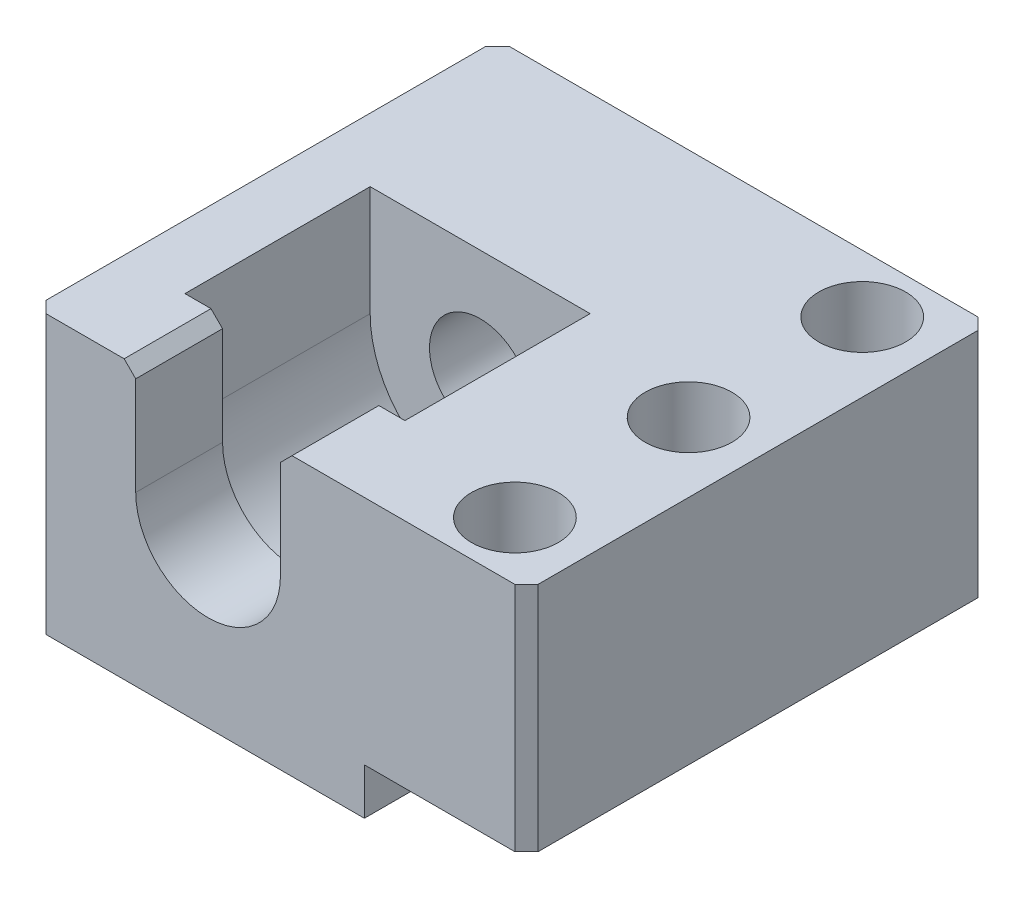
SolidWorks part; units mm, degrees
material "Q235-A"
ref_plane "Front Plane" through (0, 0, 0) normal (0, 0, 1) x (1, 0, 0)
ref_plane "Top Plane" through (0, 0, 0) normal (0, 1, 0) x (1, 0, 0)
ref_plane "Right Plane" through (0, 0, 0) normal (1, 0, 0) x (0, 0, -1)
sketch "Sketch2" plane through (0, 0, 0) normal (0, 0, 1) x (1, 0, 0)
  line L0 (-36.9628, 9.8085) -> (-36.9628, -38.1915)
  line L1 (-36.9628, -38.1915) -> (20.0372, -38.1915)
  line L2 (20.0372, -38.1915) -> (20.0372, -30.1915)
  line L3 (20.0372, -30.1915) -> (48.0372, -30.1915)
  line L4 (48.0372, -30.1915) -> (48.0372, 9.8085)
  line L5 (48.0372, 9.8085) -> (-36.9628, 9.8085)
  dimension "D1" = 85
  dimension "D2" = 8
  dimension "D3" = 48
  dimension "D4" = 57
extrude "Boss-Extrude1" add sketch "Sketch2" along normal blind 80
sketch "Sketch3" plane through (0, 0, 80) normal (0, 0, 1) x (1, 0, 0)
  line L0 (-36.9628, 9.8085) -> (-36.9628, -38.1915) construction
  line L1 (-36.9628, -38.1915) -> (20.0372, -38.1915) construction
  line L2 (-19.4628, -9.1915) -> (-19.4628, 9.8085)
  line L3 (48.0372, 9.8085) -> (-36.9628, 9.8085) construction
  line L4 (5.5372, -9.1915) -> (5.5372, 9.8085)
  line L5 (5.5372, 9.8085) -> (-19.4628, 9.8085)
  arc A0 (-19.4628, -9.1915) -> (5.5372, -9.1915) centre (-6.9628, -9.1915) ccw
  dimension "D1" = 30
  dimension "D2" = 25
  dimension "D3" = 29
extrude "Cut-Extrude1" cut sketch "Sketch3" against normal blind 15
sketch "Sketch4" plane through (0, 0, 65) normal (0, 0, 1) x (1, 0, 0)
  line L0 (-25.9628, -9.1915) -> (-25.9628, 9.8085)
  line L1 (-19.4628, 9.8085) -> (-36.9628, 9.8085) construction
  line L2 (-25.9628, 9.8085) -> (12.0372, 9.8085)
  line L3 (48.0372, 9.8085) -> (5.5372, 9.8085) construction
  line L4 (12.0372, 9.8085) -> (12.0372, -9.1915)
  arc A0 (-25.9628, -9.1915) -> (12.0372, -9.1915) centre (-6.9628, -9.1915) ccw
extrude "Cut-Extrude2" cut sketch "Sketch4" against normal blind 32
hole_wizard "M20 Tapped Hole1" positions "Sketch5" profile "Sketch6" tap size "M20" standard "GB" end condition through all
sketch "Sketch5" plane through (0, 0, 33) normal (0, 0, 1) x (1, 0, 0)
  point P0 (-6.9628, -9.1915)
sketch "Sketch6" plane through (-6.9628, -9.1915, 33) normal (1, 0, 0) x (0, -1, 0)
  line L0 (0, 0) -> (0, 33)
  line L1 (0, 33) -> (8.75, 33)
  line L2 (8.75, 33) -> (8.75, 0)
  line L5 (8.75, 0) -> (0, 0)
  line L11 (0, -6.35) -> (0, 107.95) construction
  dimension "通孔螺纹孔钻头直径" = 17.5
  dimension "通孔螺纹孔钻头深度" = 33
cosmetic thread "Cosmetic thread 1" parameters "D2"=20
sketch "Sketch7" plane through (0, 9.8085, 0) normal (0, 1, 0) x (1, 0, 0)
  line L0 (36.0372, -10) -> (36.0372, -70) construction
  line L1 (-36.9628, -80) -> (-36.9628, 0) construction
  line L2 (48.0372, -80) -> (5.5372, -80) construction
  point P6 (36.0372, -40)
  dimension "D1" = 60
  dimension "D2" = 73
  dimension "D3" = 10
hole_wizard "Hole1" positions "Sketch8" profile "Sketch9" legacy end condition through all
sketch "Sketch8" plane through (0, 9.8085, 0) normal (0, 1, 0) x (1, 0, 0)
  point P0 (36.0372, -10)
  point P3 (36.0372, -40)
  point P6 (36.0372, -70)
sketch "Sketch9" plane through (36.0372, 9.8085, 10) normal (1, 0, 0) x (0, 0, 1)
  line L0 (0, 0) -> (0, 48)
  line L1 (0, 48) -> (4.2, 48)
  line L2 (4.2, 48) -> (4.2, 20)
  line L3 (4.2, 20) -> (7.5, 20)
  line L4 (7.5, 20) -> (7.5, 0)
  line L5 (7.5, 0) -> (0, 0)
  line L6 (0, 110) -> (0, -10) construction
  dimension "直径" = 8.4
  dimension "深度" = 48
  dimension "柱坑直径" = 15
  dimension "柱坑深度" = 20
chamfer "Chamfer1" distance 2 angle 45 6 edges at (48.0372, -10.1915, 0) (48.0372, -10.1915, 80) (-36.9628, -14.1915, 0) (-36.9628, -14.1915, 80) (5.5372, 9.8085, 72.5) (-19.4628, 9.8085, 72.5)
